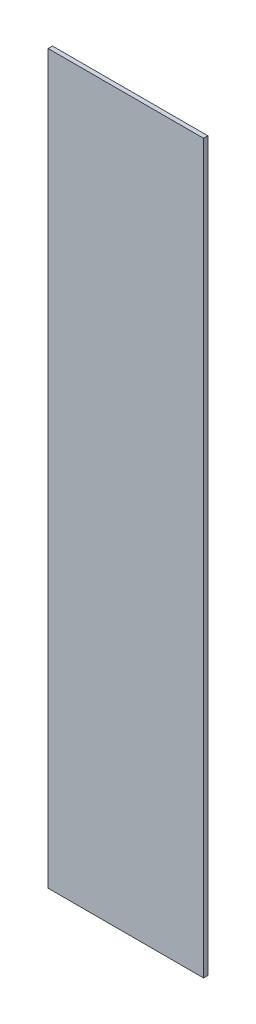
from build123d import *

# Parameters (mm, degrees)
SKETCH_1_W      = 180
SKETCH_1_H      = 842
EXTRUDE_1_DEPTH = 5


with BuildPart() as part:
    # 草图1 → 凸台-拉伸1 (new body)
    with BuildSketch(Plane.XY):
        Rectangle(SKETCH_1_W, SKETCH_1_H)
    extrude(amount=EXTRUDE_1_DEPTH)


solid = part.part
